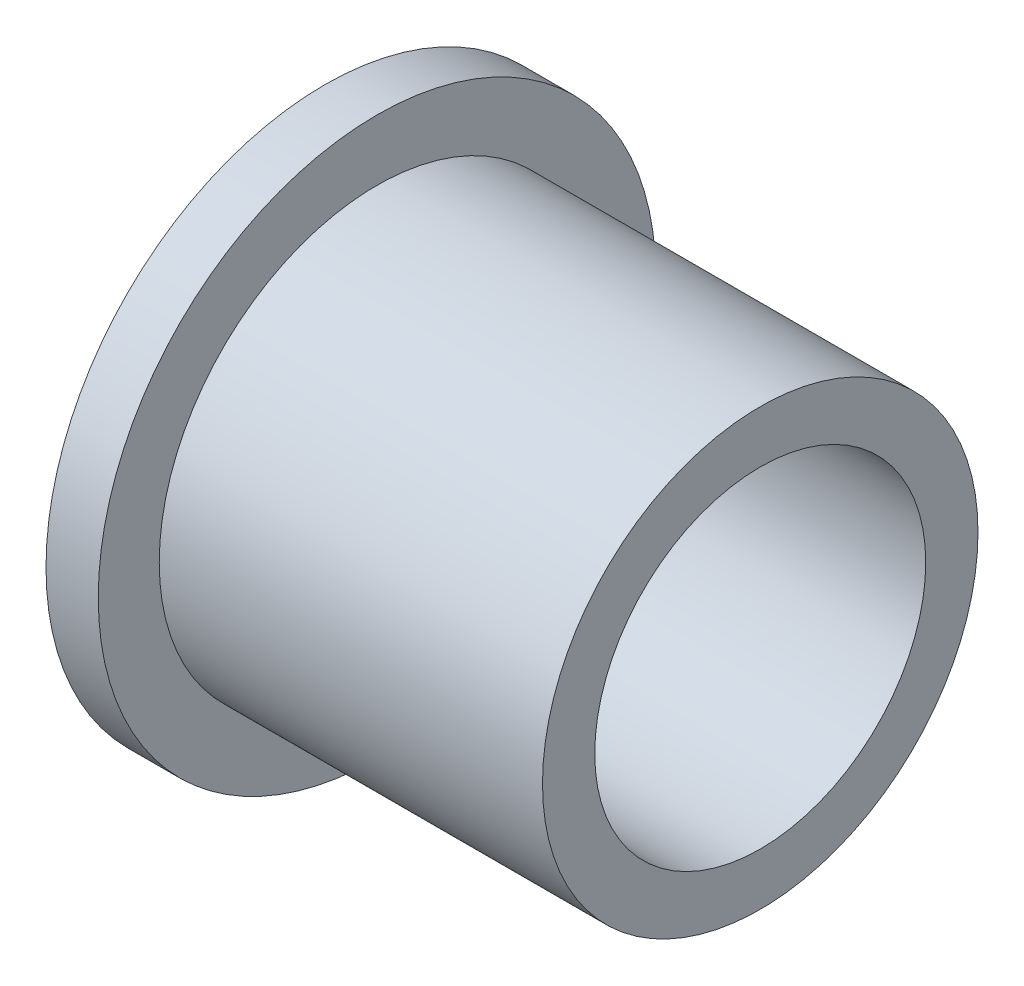
SolidWorks part; units mm, degrees
ref_plane "Front Plane" through (0, 0, 0) normal (0, 0, 1) x (1, 0, 0)
ref_plane "Top Plane" through (0, 0, 0) normal (0, 1, 0) x (1, 0, 0)
ref_plane "Right Plane" through (0, 0, 0) normal (1, 0, 0) x (0, 0, -1)
sketch "Sketch1" plane through (0, 0, 0) normal (0, 0, 1) x (1, 0, 0)
  line L0 (0, 0) -> (0, 4678.2) construction
  line L1 (0, 0) -> (5023.5102, 0) construction
  line L2 (0, 241.3) -> (0, 406.4)
  line L4 (0, 241.3) -> (635, 241.3)
  line L5 (635, 241.3) -> (635, 317.5)
  line L6 (635, 317.5) -> (76.2, 317.5)
  line L7 (76.2, 317.5) -> (76.2, 406.4)
  line L8 (76.2, 406.4) -> (0, 406.4)
  dimension "D1" = 558.8
  dimension "D2" = 635
  dimension "D3" = 406.4
  dimension "D4" = 241.3
  dimension "D5" = 76.2
revolve "Revolve1" add sketch "Sketch1" angle 360 about L1
